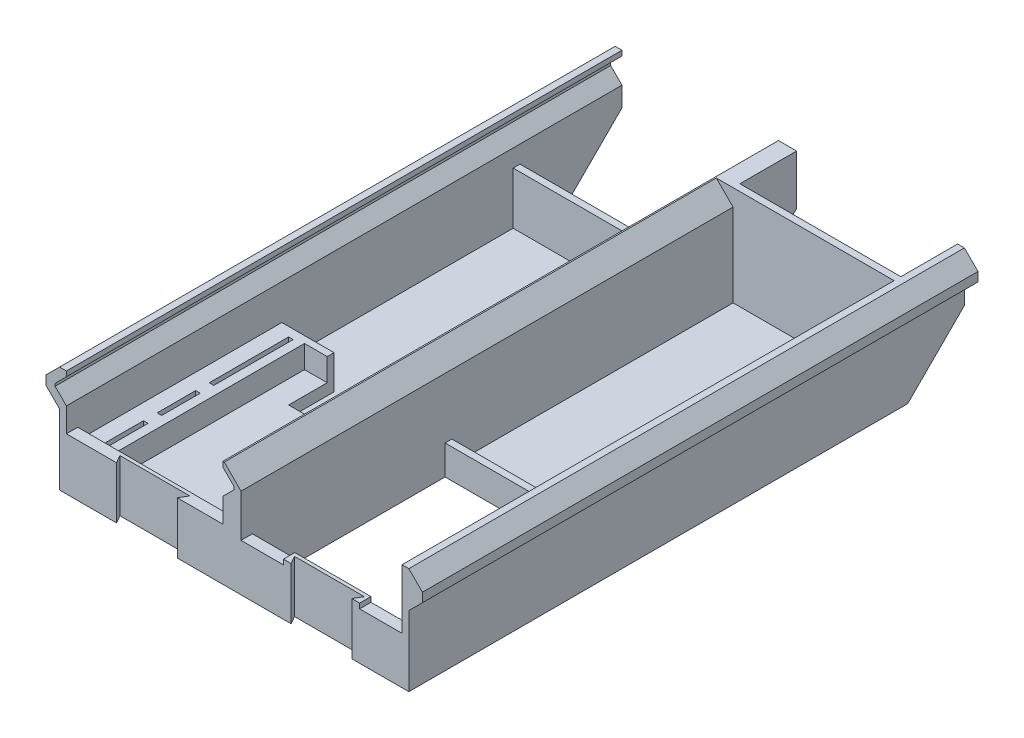
SolidWorks part; units mm, degrees
ref_plane "Front Plane" through (0, 0, 0) normal (0, 0, 1) x (1, 0, 0)
ref_plane "Top Plane" through (0, 0, 0) normal (0, 1, 0) x (1, 0, 0)
ref_plane "Right Plane" through (0, 0, 0) normal (1, 0, 0) x (0, 0, -1)
sketch "Sketch1" plane through (0, 0, 0) normal (0, 0, 1) x (1, 0, 0)
  line L0 (77, 0) -> (-77, 0)
  line L1 (-77, 0) -> (-77, 31)
  line L2 (-77, 31) -> (-83, 37)
  line L3 (-83, 37) -> (-83, 41)
  line L4 (-83, 41) -> (-77, 47)
  line L5 (-77, 47) -> (77, 47)
  line L6 (0, 47) -> (0, 0) construction
  line L7 (83, 41) -> (77, 47)
  line L8 (83, 37) -> (83, 41)
  line L9 (77, 31) -> (83, 37)
  line L10 (77, 0) -> (77, 31)
  dimension "D1" = 45
  dimension "D2" = 45
  dimension "D3" = 47
  dimension "D4" = 16
  dimension "D5" = 6
  dimension "D6" = 77
extrude "Boss-Extrude1" add sketch "Sketch1" against normal blind 200
sketch "Sketch2" plane through (0, 47, 0) normal (0, 1, 0) x (1, 0, 0)
  line L8 (-74, 3) -> (74, 3)
  line L9 (74, 3) -> (74, 197)
  line L10 (74, 197) -> (-74, 197)
  line L11 (-74, 197) -> (-74, 3)
  line L12 (-74, 3) -> (74, 3)
  line L13 (74, 3) -> (74, 197)
  line L14 (74, 197) -> (-74, 197)
  line L15 (-74, 197) -> (-74, 3)
  dimension "D1" = 3
extrude "Cut-Extrude1" cut sketch "Sketch2" against normal offset from surface (44 mm away) 3 up to face at (0, 0, -100)
sketch "Sketch4" plane through (0, 3, 0) normal (0, 1, 0) x (1, 0, 0)
  line L0 (0, 3) -> (0, 197)
  line L1 (-74, 3) -> (74, 3) construction
  line L2 (74, 197) -> (-74, 197) construction
extrude "Extrude-Thin1" add sketch "Sketch4" along normal up to surface (44 mm away) thin
sketch "Sketch5" plane through (0, 0, 0) normal (0, 0, 1) x (1, 0, 0)
  line L0 (-74, 47) -> (-74, 44.7674)
  line L1 (77, 47) -> (-77, 47) construction
  line L2 (-74, 44.7674) -> (-79, 39.7674)
  line L3 (-79, 39.7674) -> (-79, 38.6569)
  line L4 (-79, 38.6569) -> (-74, 33.6569)
  line L5 (-74, 33.6569) -> (-74, 26)
  line L6 (-74, 26) -> (-5, 26)
  line L7 (-5, 26) -> (-5, 33.6569)
  line L8 (-5, 33.6569) -> (0, 38.6569)
  line L9 (0, 38.6569) -> (0, 39.7674)
  line L10 (0, 39.7674) -> (-5, 44.7674)
  line L11 (-5, 44.7674) -> (-5, 47)
  line L12 (-73, 44.3532) -> (-78, 39.3532) construction
  line L13 (-78, 37.6569) -> (-73, 32.6569) construction
  line L14 (-6, 32.6569) -> (-1, 37.6569) construction
  line L15 (-1, 39.3532) -> (-6, 44.3532) construction
  line L16 (-74, 3) -> (-74, 47) construction
  line L17 (-78, 39.3532) -> (-78, 37.6569) construction
  line L18 (-73, 28) -> (-6, 28) construction
  line L19 (-5, 47) -> (-5, 3) construction
  line L20 (-1, 37.6569) -> (-1, 39.3532) construction
  line L31 (-77, 31) -> (-77, 0)
  line L32 (-77, 0) -> (77, 0)
  line L33 (77, 0) -> (77, 31)
  line L34 (77, 31) -> (83, 37)
  line L35 (83, 37) -> (83, 41)
  line L36 (83, 41) -> (77, 47)
  line L37 (77, 47) -> (-77, 47)
  line L38 (-77, 47) -> (-83, 41)
  line L39 (-83, 41) -> (-83, 37)
  line L40 (-83, 37) -> (-77, 31)
  line L47 (-5, 47) -> (-74, 47)
  dimension "D1" = 1
  dimension "D2" = 1
  dimension "D3" = 2
  dimension "D4" = 1
  dimension "D5" = 1
  dimension "D6" = 0
extrude "Cut-Extrude2" cut sketch "Sketch5" against normal through all
sketch "Sketch6" plane through (0, 0, -197) normal (0, 0, 1) x (1, 0, 0)
  line L0 (-4.4042, 47) -> (3, 39.5958)
  line L1 (77, 47) -> (-5, 47) construction
  line L2 (3, 39.5958) -> (3, 47) construction
  line L3 (3, 47) -> (-4.4042, 47)
  line L4 (0, 39.7674) -> (-5, 44.7674) construction
  line L5 (3, 47) -> (3, 3) construction
  line L6 (3, 39.5958) -> (74, 39.5958)
  line L7 (74, 3) -> (74, 47) construction
  line L8 (74, 39.5958) -> (74, 47)
  line L9 (74, 47) -> (3, 47)
  dimension "D1" = 2
extrude "Cut-Extrude3" cut sketch "Sketch6" along normal through all
other "Move Face1" face at (-39.5, 14.5, -3) face at (38.5, 21.2979, -3) parameters "D1"=2
sketch "Sketch7" plane through (0, 0, 0) normal (0, -1, 0) x (1, 0, 0)
  line L0 (-51.8834, 0) -> (-53.9041, -3.5)
  line L1 (-72.5, 0) -> (72.5, 0) construction
  line L2 (-53.9041, -3.5) -> (-23.0959, -3.5)
  line L3 (-23.0959, -3.5) -> (-25.1166, 0)
  line L4 (-25.1166, 0) -> (-51.8834, 0)
  line L5 (-53.5, -3) -> (-51.7679, 0) construction
  line L6 (-23.5, -3) -> (-25.2321, 0) construction
  line L7 (-23.5, -3) -> (-53.5, -3) construction
  line L8 (0, 0) -> (0, 21.1047) construction
  line L9 (25.1166, 0) -> (51.8834, 0)
  line L10 (23.0959, -3.5) -> (25.1166, 0)
  line L11 (53.9041, -3.5) -> (23.0959, -3.5)
  line L12 (51.8834, 0) -> (53.9041, -3.5)
  dimension "D1" = 0.1
  dimension "D2" = 0.1
  dimension "D3" = 0.5
extrude "Cut-Extrude4" cut sketch "Sketch7" against normal through all
sketch "Sketch8" plane through (0, 39.5958, 0) normal (0, 1, 0) x (1, 0, 0)
  line L8 (25.1166, 0) -> (23.0959, 3.5)
  line L9 (23.0959, 3.5) -> (53.9041, 3.5)
  line L10 (53.9041, 3.5) -> (51.8834, 0)
  line L11 (51.8834, 0) -> (74, 0)
  line L12 (74, 0) -> (74, 5)
  line L13 (74, 5) -> (3, 5)
  line L14 (3, 5) -> (3, 0)
  line L15 (3, 0) -> (25.1166, 0)
  line L16 (25.1166, 0) -> (23.0959, 3.5)
  line L17 (23.0959, 3.5) -> (53.9041, 3.5)
  line L18 (53.9041, 3.5) -> (51.8834, 0)
  line L19 (51.8834, 0) -> (74, 0)
  line L20 (74, 0) -> (74, 5)
  line L21 (74, 5) -> (3, 5)
  line L22 (3, 5) -> (3, 0)
  line L23 (3, 0) -> (25.1166, 0)
  line L24 (-53.9041, 3.5) -> (-23.0959, 3.5)
  line L25 (-23.0959, 3.5) -> (-25.1166, 0)
  line L26 (-25.1166, 0) -> (-5, 0)
  line L27 (-5, 0) -> (-5, 5)
  line L28 (-5, 5) -> (-74, 5)
  line L29 (-74, 5) -> (-74, 0)
  line L30 (-74, 0) -> (-51.8834, 0)
  line L31 (-51.8834, 0) -> (-53.9041, 3.5)
  line L32 (-53.9041, 3.5) -> (-23.0959, 3.5)
  line L33 (-23.0959, 3.5) -> (-25.1166, 0)
  line L34 (-25.1166, 0) -> (-5, 0)
  line L35 (-5, 0) -> (-5, 5)
  line L36 (-5, 5) -> (-74, 5)
  line L37 (-74, 5) -> (-74, 0)
  line L38 (-74, 0) -> (-51.8834, 0)
  line L39 (-51.8834, 0) -> (-53.9041, 3.5)
  dimension "D1" = 0
  dimension "D2" = 0
extrude "Cut-Extrude5" cut sketch "Sketch8" against normal up to vertex (16.5958 mm away)
other "Move Face2" face at (-21.5455, 35.0771, -200) parameters "D1"=45
other "Move Face3" face at (29.9192, 27.9192, -197) parameters "D1"=20
sketch "Sketch9" plane through (0, 0, -245) normal (0, 0, -1) x (-1, 0, 0)
  line L0 (77, 0) -> (-77, 0) construction
  line L1 (-74, 47) -> (-3, 47)
  line L2 (-74, 47) -> (-74, 0)
  line L3 (-74, 0) -> (-3, 0)
  line L4 (-3, 47) -> (-3, 0)
  line L5 (-3, 39.5958) -> (-3, 3) construction
extrude "Cut-Extrude6" cut sketch "Sketch9" against normal offset from surface (25 mm away) 3
sketch "Sketch10" plane through (0, 0, -245) normal (0, 0, -1) x (-1, 0, 0)
  line L0 (77, 0) -> (-3, 0) construction
  line L1 (5, 26) -> (74, 26)
  line L2 (5, 26) -> (5, 0)
  line L3 (5, 0) -> (74, 0)
  line L4 (74, 26) -> (74, 0)
  line L5 (74, 33.6569) -> (74, 26) construction
extrude "Cut-Extrude7" cut sketch "Sketch10" against normal offset from surface (45 mm away) 3 up to face at (-39.5, 14.5, -197)
sketch "Sketch11" plane through (0, 0, -245) normal (0, 0, -1) x (-1, 0, 0)
  line L0 (5, 0) -> (5, 30.6569)
  line L1 (5, 0) -> (5, 33.6569) construction
  line L2 (5, 30.6569) -> (0, 25.6569)
  line L3 (0, 25.6569) -> (0, 0)
  line L4 (5, 0) -> (-3, 0) construction
  line L5 (0, 0) -> (5, 0)
  line L6 (-3, 0) -> (-3, 47) construction
  dimension "D1" = 3
  dimension "D2" = 45
  dimension "D3" = 3
extrude "Cut-Extrude8" cut sketch "Sketch11" against normal up to surface (45 mm away) up to face at (-39.5, 13, -200)
chamfer "Chamfer1" distance 25 angle 45 3 edges at (-75.5, 0, -245) (1.5, 0, -245) (75.5, 0, -245)
sketch "Sketch12" plane through (0, 3, 0) normal (0, 1, 0) x (1, 0, 0)
  line L0 (74, 0) -> (74, 217) construction
  line L1 (3, 5) -> (74, 5)
  line L2 (3, 5) -> (3, 90)
  line L3 (3, 90) -> (74, 90)
  line L4 (74, 5) -> (74, 90)
  dimension "D1" = 85
extrude "Cut-Extrude9" cut sketch "Sketch12" against normal up to next
sketch "Sketch13" plane through (0, 3, 0) normal (0, 1, 0) x (1, 0, 0)
  line L0 (74, 0) -> (74, 217) construction
  line L1 (3, 90) -> (74, 90)
  line L2 (3, 90) -> (3, 93)
  line L3 (3, 93) -> (74, 93)
  line L4 (74, 90) -> (74, 93)
  dimension "D1" = 3
extrude "Boss-Extrude2" add sketch "Sketch13" along normal blind 10
sketch "Sketch14" plane through (0, 23, 0) normal (0, 1, 0) x (1, 0, 0)
  line L0 (74, 5) -> (3, 5) construction
  line L1 (3, 0) -> (21.7, 0)
  line L2 (3, 0) -> (3, 5)
  line L3 (3, 5) -> (21.7, 5)
  line L4 (21.7, 0) -> (21.7, 5)
  line L5 (21.2, 0.5) -> (21.2, 5.2) construction
  line L6 (74, 0) -> (55.3, 0)
  line L7 (74, 0) -> (74, 5)
  line L8 (74, 5) -> (55.3, 5)
  line L9 (55.3, 0) -> (55.3, 5)
  line L10 (55.8, 5.2) -> (55.8, 0.5) construction
  dimension "D1" = 0.5
  dimension "D2" = 0.5
extrude "Cut-Extrude10" cut sketch "Sketch14" against normal blind 2.2
sketch "Sketch15" plane through (0, 3, 0) normal (0, 1, 0) x (1, 0, 0)
  line L0 (-5, 0) -> (-5, 245) construction
  line L1 (-74, 5) -> (-5, 5)
  line L2 (-74, 5) -> (-74, 95)
  line L3 (-74, 95) -> (-5, 95)
  line L4 (-5, 5) -> (-5, 95)
  dimension "D1" = 90
extrude "Boss-Extrude3" add sketch "Sketch15" along normal blind 15
sketch "Sketch16" plane through (0, 18, 0) normal (0, 1, 0) x (1, 0, 0)
  line L1 (-5, 5) -> (-61, 5)
  line L2 (-5, 5) -> (-5, 92)
  line L3 (-5, 92) -> (-61, 92)
  line L4 (-61, 5) -> (-61, 92)
  dimension "D1" = 56
  dimension "D2" = 87
extrude "Cut-Extrude11" cut sketch "Sketch16" against normal blind 10
sketch "Sketch17" plane through (0, 18, 0) normal (0, 1, 0) x (1, 0, 0)
  line L0 (-5, 92) -> (-61, 92) construction
  line L1 (-5, 95) -> (-74, 95) construction
  line L2 (-51, 109) -> (-15, 109)
  line L3 (-51, 109) -> (-51, 75)
  line L4 (-51, 75) -> (-15, 75)
  line L5 (-15, 109) -> (-15, 75)
  line L6 (-51, 109) -> (-15, 75) construction
  line L7 (-51, 75) -> (-15, 109) construction
  line L8 (-61, 92) -> (-61, 5) construction
  point P2 (-33, 92)
  dimension "D1" = 20
  dimension "D2" = 10
extrude "Cut-Extrude12" cut sketch "Sketch17" against normal up to surface (15 mm away) up to face at (-39.5, 3, -146)
sketch "Sketch18" plane through (0, 18, 0) normal (0, 1, 0) x (1, 0, 0)
  line L0 (-65, 10) -> (-65, 27)
  line L1 (-61, 92) -> (-61, 5) construction
  line L2 (-65, 33) -> (-65, 50)
  line L3 (-65, 56) -> (-65, 91)
  line L4 (-5, 5) -> (-74, 5) construction
  dimension "D1" = 17
  dimension "D2" = 4
  dimension "D3" = 5
  dimension "D4" = 6
  dimension "D5" = 6
  dimension "D6" = 35
extrude "Cut-Extrude-Thin1" cut sketch "Sketch18" against normal blind 7 thin thin type one direction reverse wall 2
other "Move Face4" face at (-66, 11, -73.5) parameters "D1"=3
